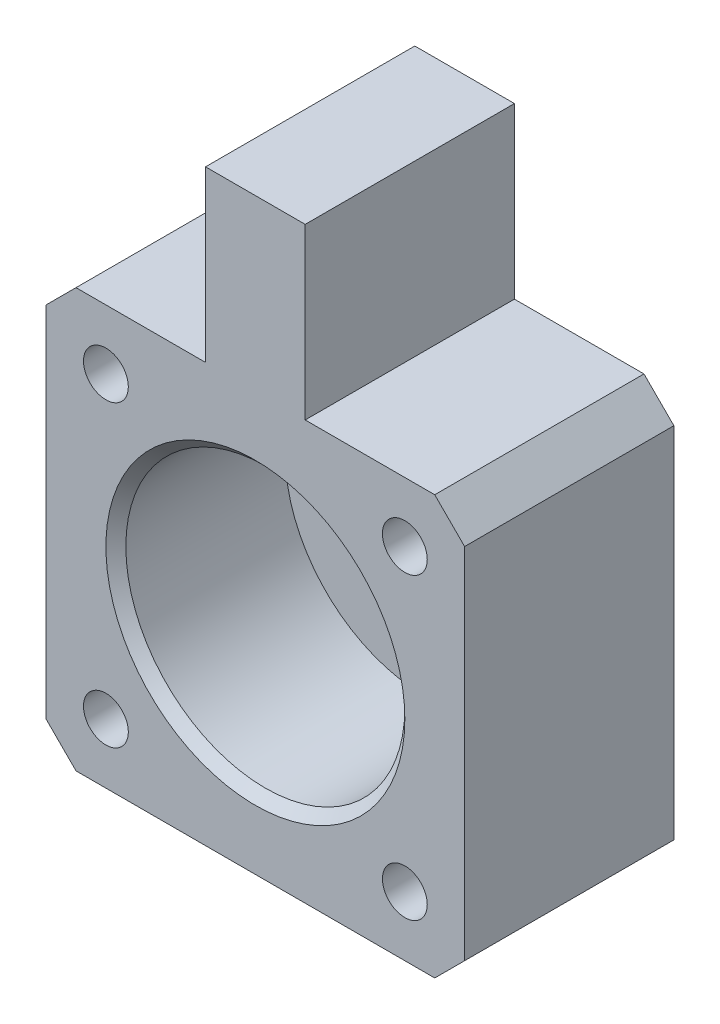
from build123d import *

# Parameters (mm, degrees)
SKETCH_1_W                = 42
SKETCH_1_H                = 42
EXTRUDE_1_DEPTH           = 12
SKETCH_2_R                = 14
CUT_EXTRUDE_1_DEPTH       = 8
SKETCH_3_R                = 8
CUT_EXTRUDE_2_DEPTH       = 50.629250448
CHAMFER_1_SIZE            = 3
HOLE_WIZARD_2_D           = 4.5
HOLE_WIZARD_2_CBORE_D     = 8
HOLE_WIZARD_2_CBORE_DEPTH = 4.6
EXTRUDE_START             = 9
SKETCH_10_R               = 2.25
SKETCH_10_R_2             = 14
EXTRUDE_2_DEPTH           = 9
SKETCH_11_W               = 10
SKETCH_11_H               = 17
EXTRUDE_3_DEPTH           = 21
HOLE_WIZARD_M3_1_D        = 2.5
HOLE_WIZARD_M3_1_DEPTH    = 7
HOLE_WIZARD_M3_1_TIP      = 0.751075774
CHAMFER_2_SIZE            = 1


with BuildPart() as part:
    # 草图1 → 凸台-拉伸1 (new body)
    with BuildSketch(Plane.XY):
        with Locations((0, 23.25)):
            Rectangle(SKETCH_1_W, SKETCH_1_H)
    extrude(amount=EXTRUDE_1_DEPTH)

    # 草图2 → 切除-拉伸1 (cut)
    with BuildSketch(Plane.XY.offset(12)):
        with Locations((0, 23.25)):
            Circle(SKETCH_2_R)
    extrude(amount=-CUT_EXTRUDE_1_DEPTH, mode=Mode.SUBTRACT)

    # 草图3 → 切除-拉伸2 (cut, through all)
    with BuildSketch(Plane.XY.offset(4)):
        with Locations((0, 23.25)):
            Circle(SKETCH_3_R)
    extrude(amount=-CUT_EXTRUDE_2_DEPTH, mode=Mode.SUBTRACT)

    # 倒角1
    chamfer_1_edges = [part.edges().sort_by_distance(p)[0] for p in [
        (21, 2.25, 6),
        (-21, 2.25, 6),
        (-21, 44.25, 6),
        (21, 44.25, 6),
    ]]
    chamfer(chamfer_1_edges, length=CHAMFER_1_SIZE)

    # 打孔尺寸根据内六角圆柱头螺钉的类型2 (through all)
    with Locations(Plane(origin=(0, 0, 0), x_dir=(-1, 0, 0), z_dir=(0, 0, -1))):
        with Locations((-15, 38.25), (15, 38.25), (15, 8.25), (-15, 8.25)):
            CounterBoreHole(HOLE_WIZARD_2_D / 2, HOLE_WIZARD_2_CBORE_D / 2, HOLE_WIZARD_2_CBORE_DEPTH)

    # 草图10 → 凸台-拉伸2 (add)
    with BuildSketch(Plane.XY.offset(12).offset(EXTRUDE_START)):
        Polygon((-18, 2.25), (18, 2.25), (21, 5.25), (21, 41.25), (18, 44.25), (-18, 44.25), (-21, 41.25), (-21, 5.25), align=None)
        with Locations(Location((-15, 38.25, 0), (0, 0, 180))):
            Circle(SKETCH_10_R, mode=Mode.SUBTRACT)
        with Locations((0, 23.25)):
            Circle(SKETCH_10_R_2, mode=Mode.SUBTRACT)
        with Locations(Location((15, 38.25, 0), (0, 0, 180))):
            Circle(SKETCH_10_R, mode=Mode.SUBTRACT)
        with Locations(Location((15, 8.25, 0), (0, 0, 180))):
            Circle(SKETCH_10_R, mode=Mode.SUBTRACT)
        with Locations(Location((-15, 8.25, 0), (0, 0, 180))):
            Circle(SKETCH_10_R, mode=Mode.SUBTRACT)
    extrude(amount=-EXTRUDE_2_DEPTH)

    # 草图11 → 凸台-拉伸3 (add)
    with BuildSketch(Plane(origin=(0, 0, 0), x_dir=(-1, 0, 0), z_dir=(0, 0, -1))):
        with Locations((0, 52.75)):
            Rectangle(SKETCH_11_W, SKETCH_11_H)
    extrude(amount=-EXTRUDE_3_DEPTH)

    # M3 螺纹孔1
    with Locations(Plane(origin=(0, 0, 0), x_dir=(-1, 0, 0), z_dir=(0, 0, -1))):
        with Locations((0, 57.75), (0, 39.25)):
            Hole(HOLE_WIZARD_M3_1_D / 2, depth=HOLE_WIZARD_M3_1_DEPTH)
            with Locations((0, 0, -(HOLE_WIZARD_M3_1_DEPTH + HOLE_WIZARD_M3_1_TIP / 2))):  # 118° drill point
                Cone(0, HOLE_WIZARD_M3_1_D / 2, HOLE_WIZARD_M3_1_TIP, mode=Mode.SUBTRACT)

    # 倒角2
    chamfer_2_edges = [part.edges().sort_by_distance(p)[0] for p in [
        (-14, 23.25, 21),
    ]]
    chamfer(chamfer_2_edges, length=CHAMFER_2_SIZE)


solid = part.part
